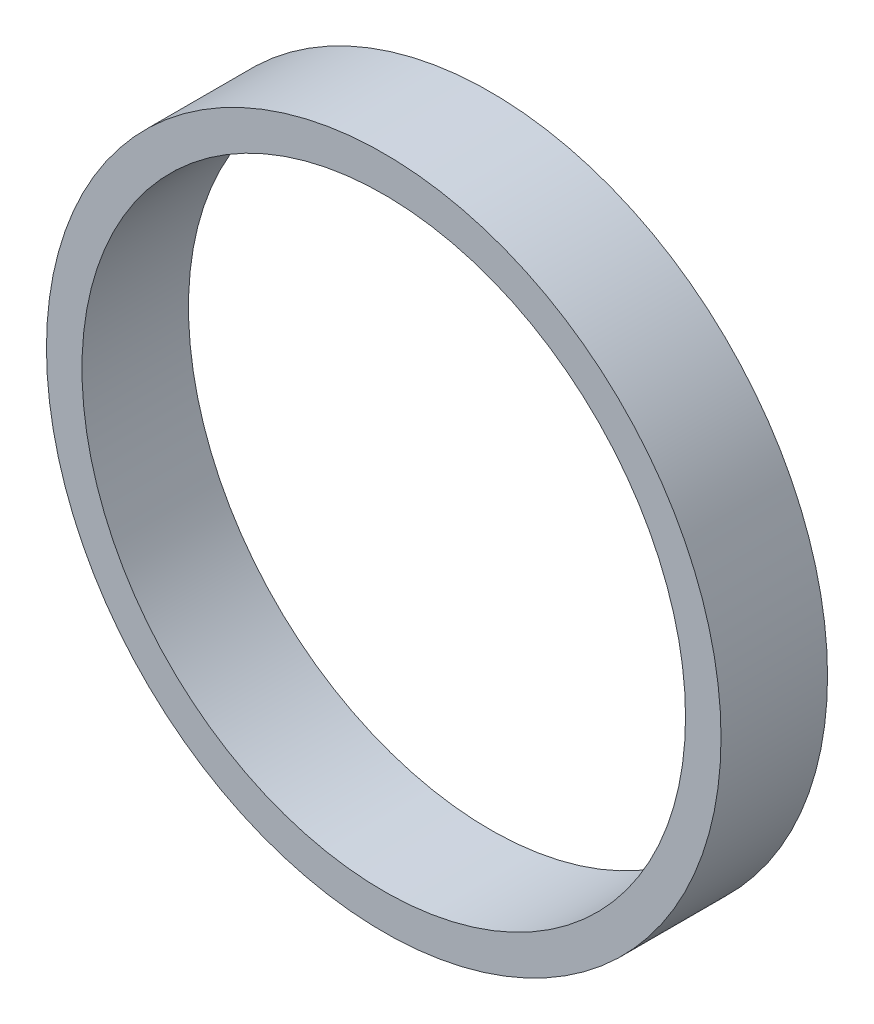
SolidWorks part; units mm, degrees
ref_plane "Front Plane" through (0, 0, 0) normal (0, 0, 1) x (1, 0, 0)
ref_plane "Top Plane" through (0, 0, 0) normal (0, 1, 0) x (1, 0, 0)
ref_plane "Right Plane" through (0, 0, 0) normal (1, 0, 0) x (0, 0, -1)
other "Configuration Table"
sketch "Sketch2" plane through (0, 0, 0) normal (0, 0, 1) x (1, 0, 0)
  circle A0 centre (0, 0) radius 95
  circle A3 centre (0, 0) radius 85
  dimension "D1" = 190
  dimension "D2" = 170
extrude "Boss-Extrude1" add sketch "Sketch2" along normal blind 30
